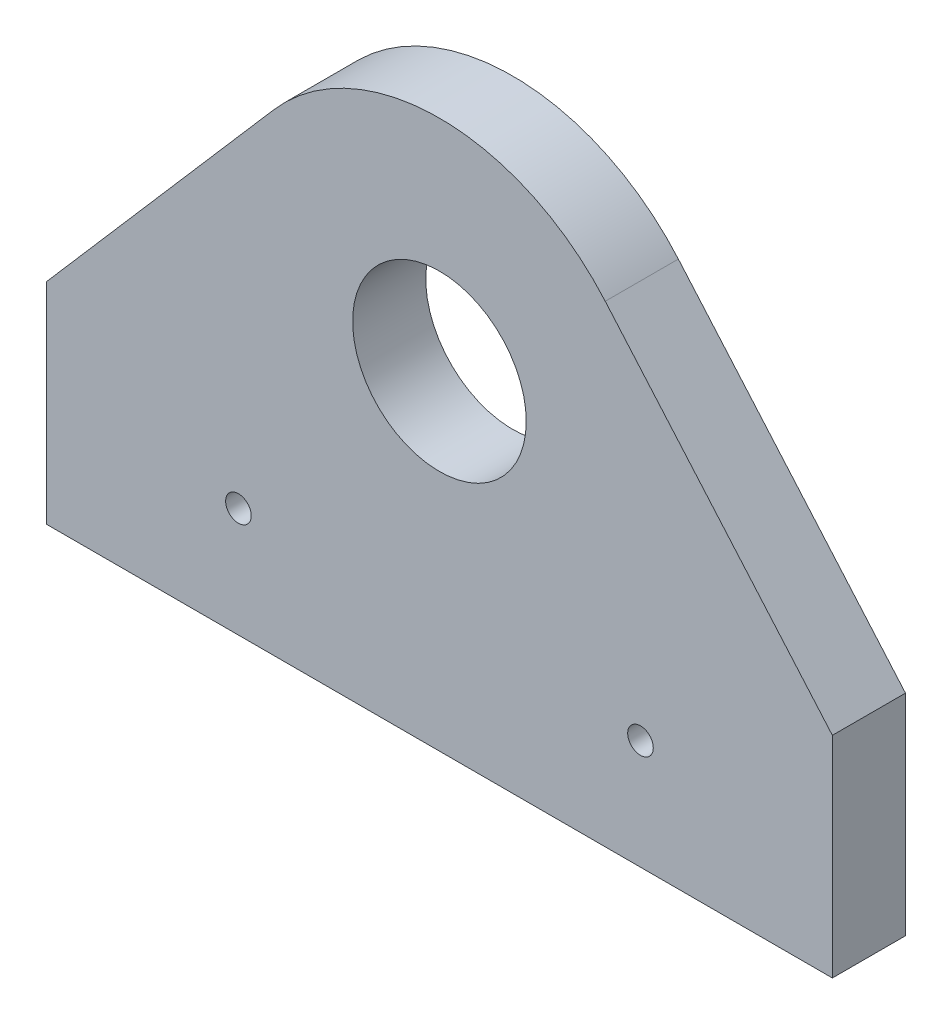
from build123d import *

# Parameters (mm, degrees)
BOSS_EXTRUDE1_DEPTH = 40
SKETCH2_R           = 47.5
CUT_EXTRUDE1_DEPTH  = 284.240180765
M16_TAPPED_HOLE1_D  = 14


with BuildPart() as part:
    # Sketch1 → Boss-Extrude1 (new body)
    with BuildSketch(Plane.XY):
        with BuildLine():
            Line((-215, -180), (215, -180))
            Line((215, -180), (215, -65))
            Line((215, -65), (90.722959932, 78.545175161))
            ThreePointArc((90.722959932, 78.545175161), (0, 120), (-90.722959932, 78.545175161))
            Line((-90.722959932, 78.545175161), (-215, -65))
            Line((-215, -65), (-215, -180))
        make_face()
    extrude(amount=BOSS_EXTRUDE1_DEPTH)

    # Sketch2 → Cut-Extrude1 (cut, through all)
    with BuildSketch(Plane.XY.offset(40)):
        Circle(SKETCH2_R)
    extrude(amount=-CUT_EXTRUDE1_DEPTH, mode=Mode.SUBTRACT)

    # M16 Tapped Hole1 (through all)
    with Locations(Plane.XY.offset(40)):
        with Locations((-110, -120), (110, -120)):
            Hole(M16_TAPPED_HOLE1_D / 2)


solid = part.part
